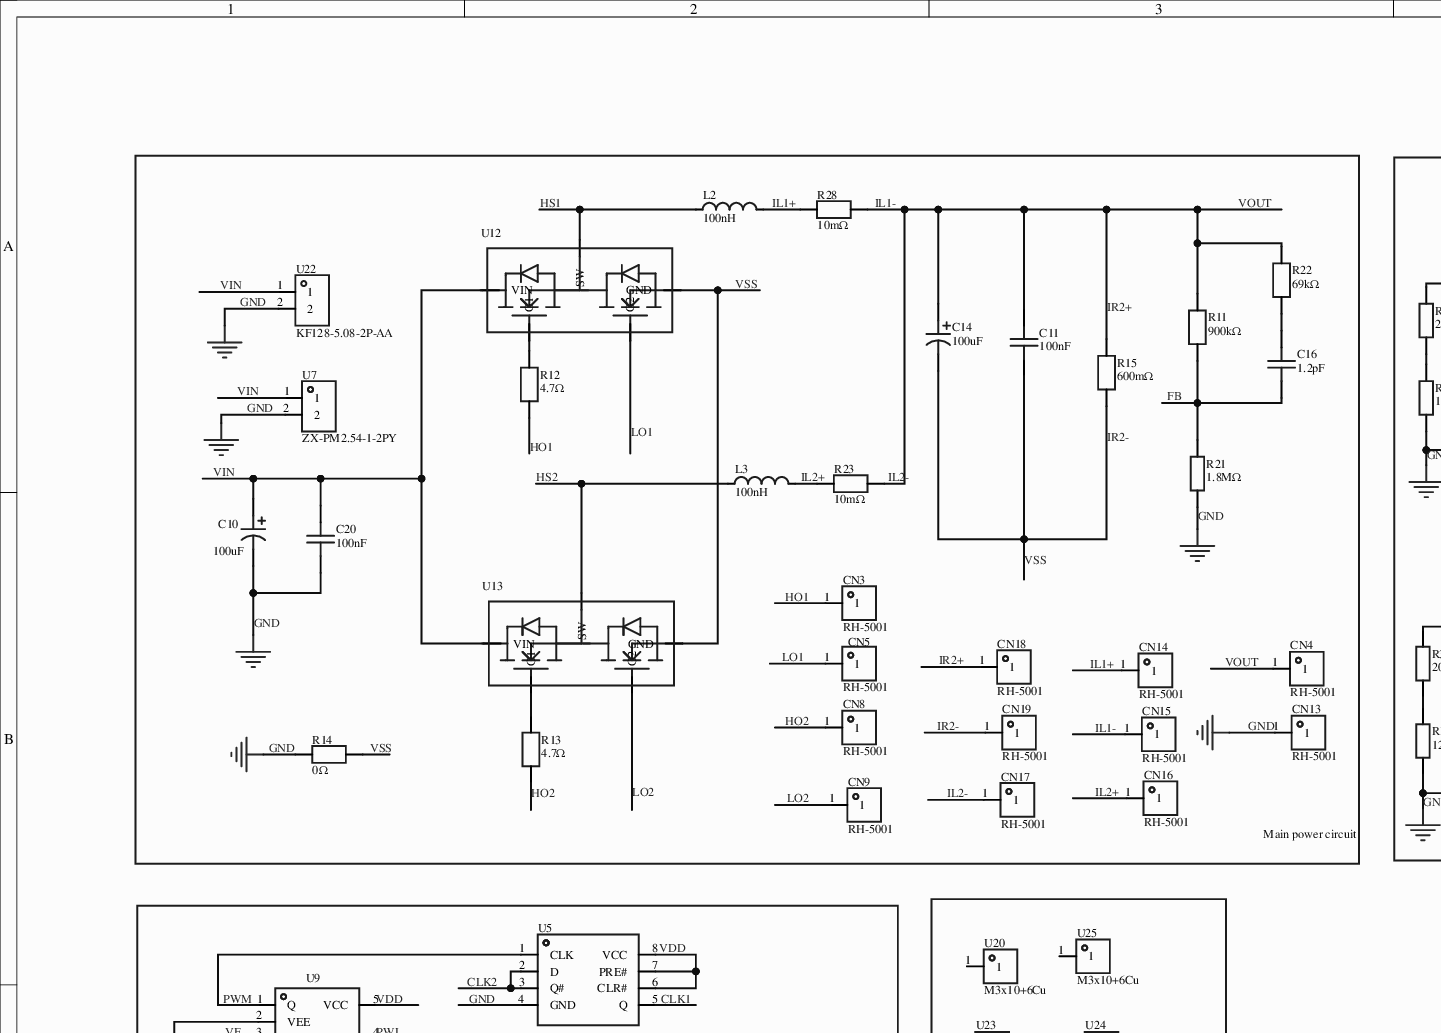
[diagram p0: MISC53275-3.schdoc, top left]
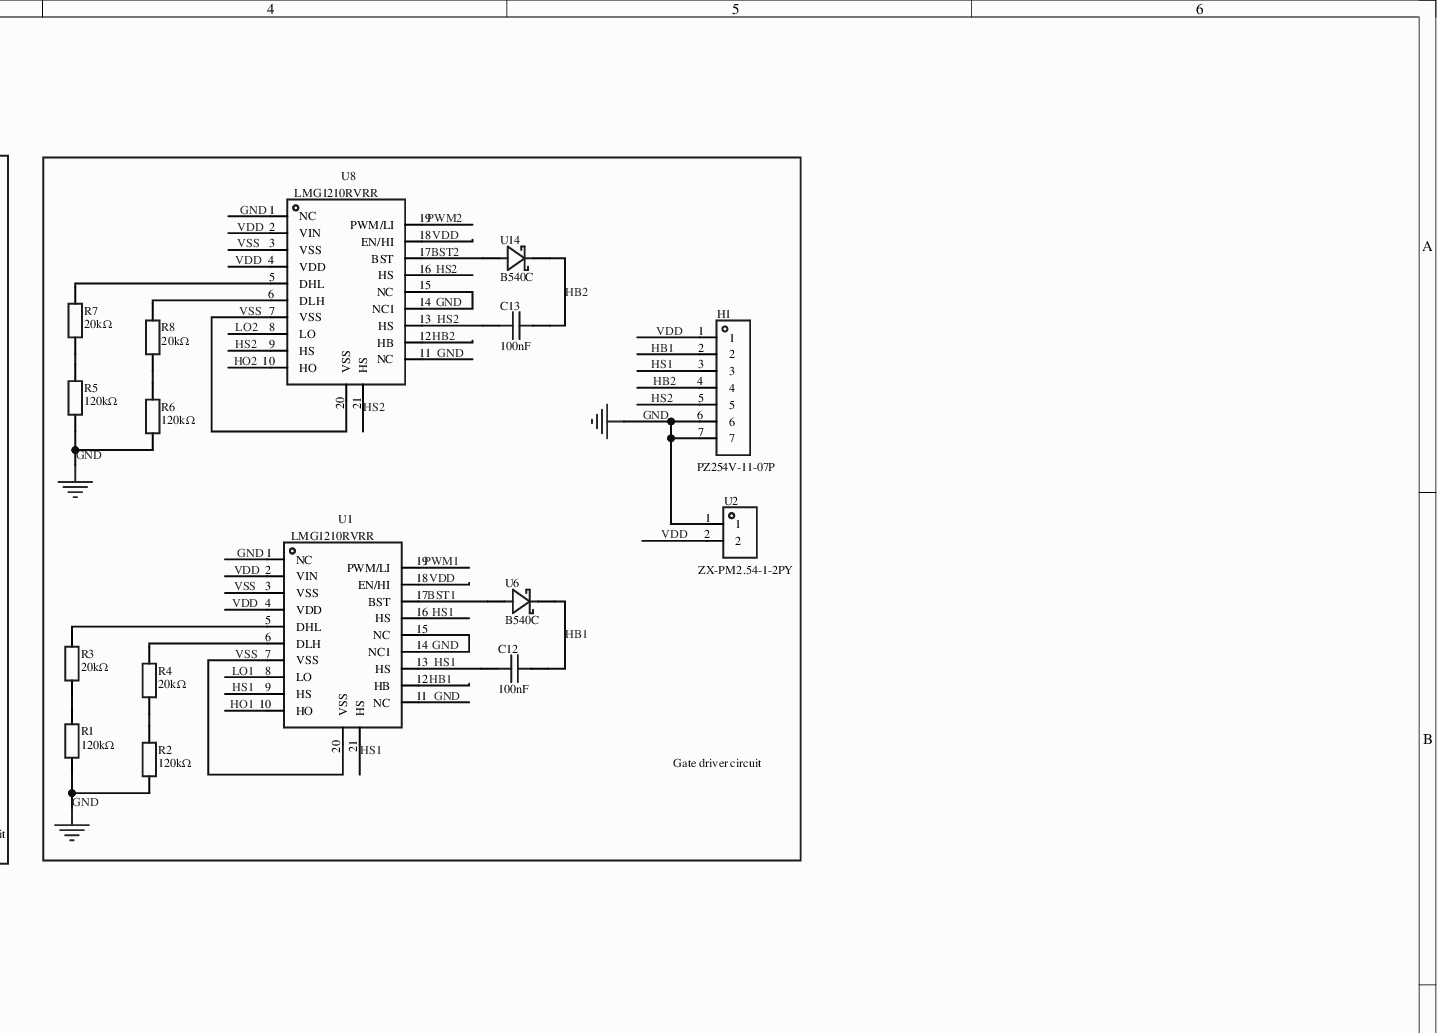
[diagram p1: MISC53275-3.schdoc, top right]
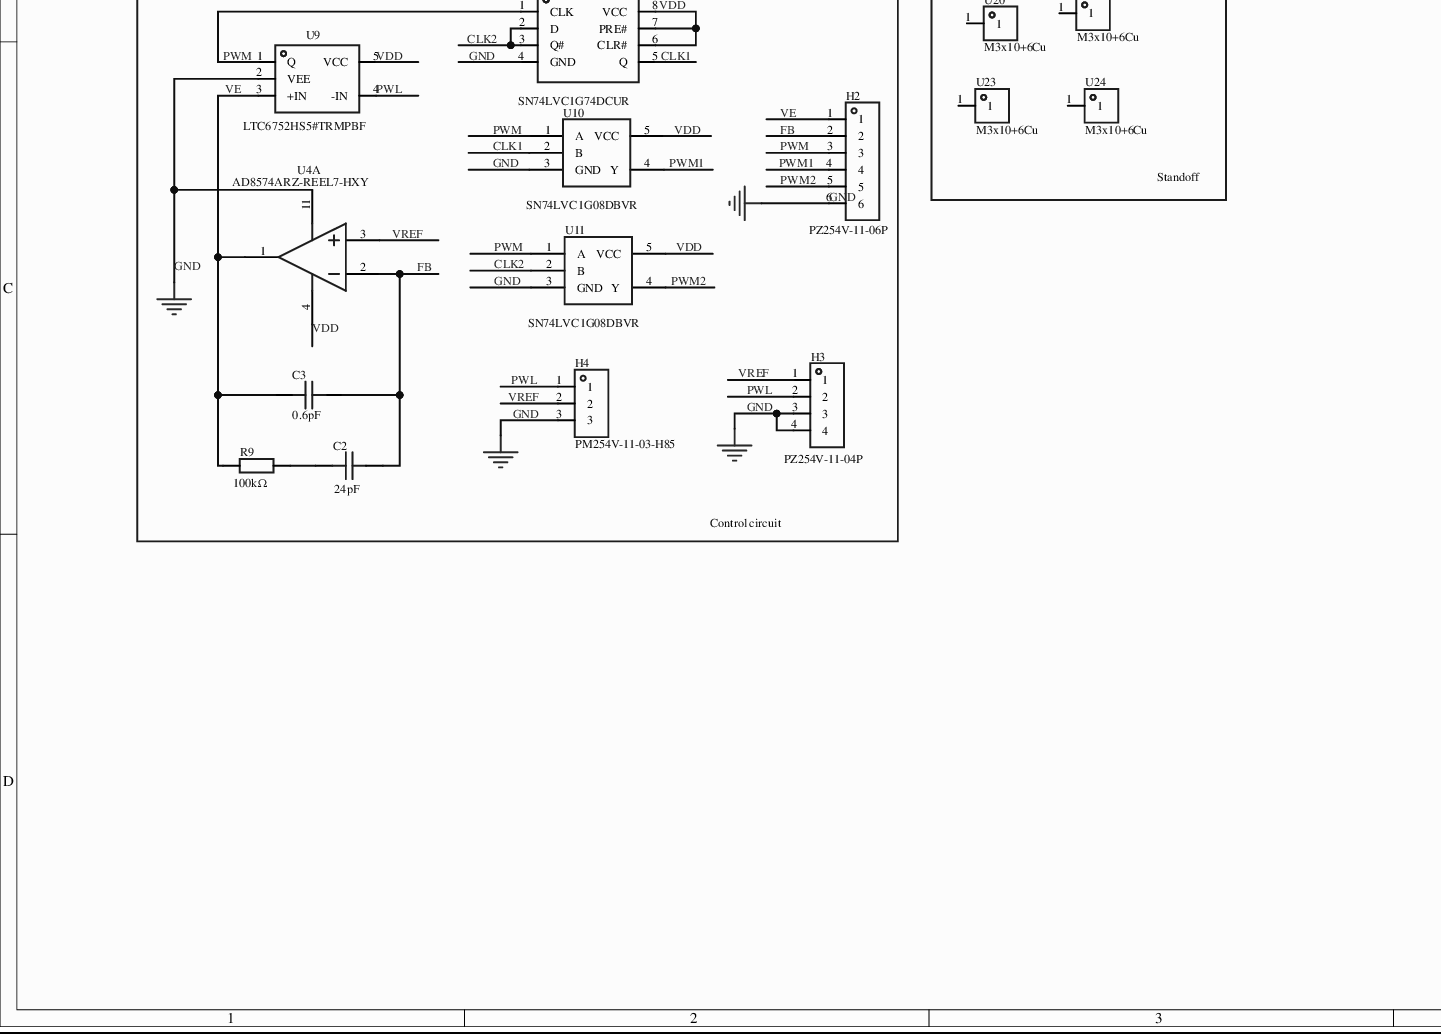
[diagram p2: MISC53275-3.schdoc, bottom left]
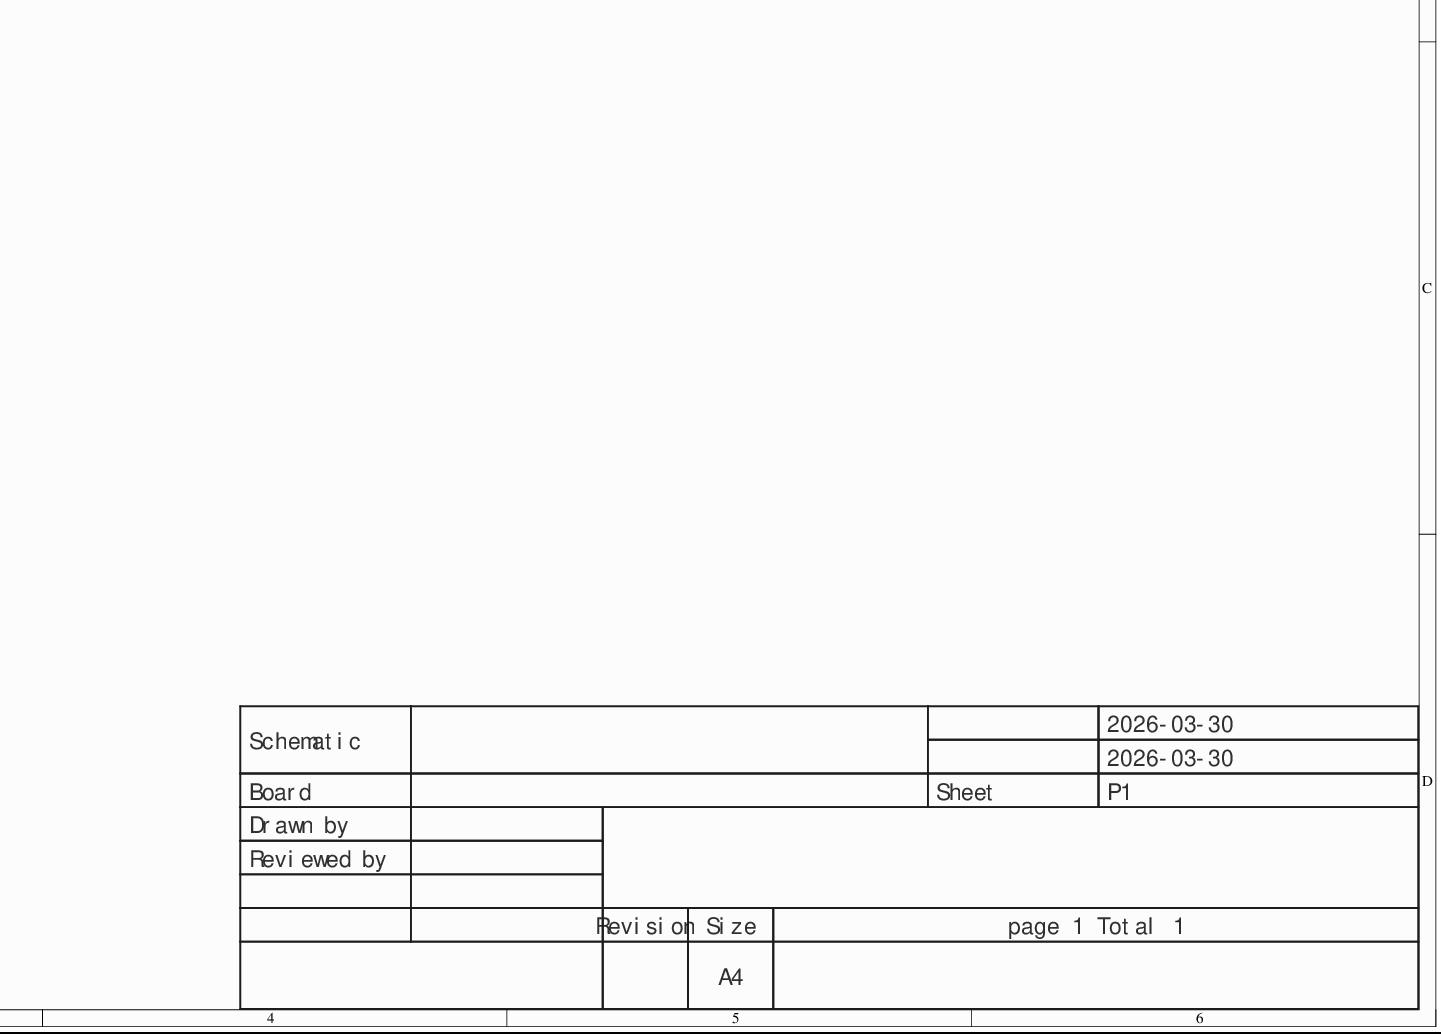
[diagram p3: MISC53275-3.schdoc, bottom right]
# Altium project MISC53275-2.PrjPcb
1 sheet, 63 parts. Net scope: global (net labels, ports and power ports of the same name join across sheets).
Board file: MISC53275.pcbdoc

## Sheet MISC53275-3.schdoc
size 420 x 297 mm; Version: V1.0; @Project Name: MISC53275; @Update Date: 2026-03-30; @Create Date: 2026-03-30; @Board Name: MISC53275; @Create Time: 11:56:40; @Page Count: 1; @Page No: 1; @Schematic Name: MISC53275; @Update Time: 11:56:40; Size: A4

### Parts
C2  24pF  [C0805]
C3  0.6pF  [C0603]
C10  100uF  [CAP-SMD_BD6.3-L6.6-W6.6-LS7.3-FD-H7.7]
C11  100nF  [CAP-SMD_L2.0-W1.25]
C12  100nF  [CAP-SMD_L2.0-W1.25]
C13  100nF  [CAP-SMD_L2.0-W1.25]
C14  100uF  [CAP-SMD_BD6.3-L6.6-W6.6-RD]
C16  1.2pF  [C0805]
C20  100nF  [CAP-SMD_L2.0-W1.25]
CN3  RH-5001  [TEST-TH_BD2.54-P1.4_BLACK]
CN4  RH-5001  [TEST-TH_BD2.54-P1.4_BLACK]
CN5  RH-5001  [TEST-TH_BD2.54-P1.4_BLACK]
CN8  RH-5001  [TEST-TH_BD2.54-P1.4_BLACK]
CN9  RH-5001  [TEST-TH_BD2.54-P1.4_BLACK]
CN13  RH-5001  [TEST-TH_BD2.54-P1.4_BLACK]
CN14  RH-5001  [TEST-TH_BD2.54-P1.4_BLACK]
CN15  RH-5001  [TEST-TH_BD2.54-P1.4_BLACK]
CN16  RH-5001  [TEST-TH_BD2.54-P1.4_BLACK]
CN17  RH-5001  [TEST-TH_BD2.54-P1.4_BLACK]
CN18  RH-5001  [TEST-TH_BD2.54-P1.4_BLACK]
CN19  RH-5001  [TEST-TH_BD2.54-P1.4_BLACK]
H1  PZ254V-11-07P  [HDR-TH_7P-P2.54-V-M]
H2  PZ254V-11-06P  [HDR-TH_6P-P2.54-V-M]
H3  PZ254V-11-04P  [HDR-TH_4P-P2.54-V-M]
H4  PM254V-11-03-H85  [HDR-TH_3P-P2.54-V-F]
L2  100nH  [IND-SMD_L2.3-W1.8]
L3  100nH  [IND-SMD_L2.3-W1.8]
R1  120kΩ  [R0805]
R2  120kΩ  [R0805]
R3  20kΩ  [R0805]
R4  20kΩ  [R0805]
R5  120kΩ  [R0805]
R6  120kΩ  [R0805]
R7  20kΩ  [R0805]
R8  20kΩ  [R0805]
R9  100kΩ  [R0805]
R11  900kΩ  [R1206]
R12  4.7Ω  [R0805]
R13  4.7Ω  [R0805]
R14  0Ω  [R1206]
R15  600mΩ  [R1206]
R21  1.8MΩ  [R0805]
R22  69kΩ  [R0603]
R23  10mΩ  [R0805]
R28  10mΩ  [R0805]
U1  LMG1210RVRR  [WQFN-19_L4.0-W3.0-P0.50-BL-EP_LMG1210RVRR]
U2  ZX-PM2.54-1-2PY  [HDR-TH_2P-P2.54-V-F]
U4  AD8574ARZ-REEL7-HXY  [SOP-14_L8.7-W3.9-P1.27-LS6.0-BL]  (part A of 4)
U5  SN74LVC1G74DCUR  [SSOP-8_L2.0-W2.3-P0.50-LS3.1-BR]
U6  B540C  [SMC_L6.9-W5.9-LS7.9-RD]
U7  ZX-PM2.54-1-2PY  [HDR-TH_2P-P2.54-V-F]
U8  LMG1210RVRR  [WQFN-19_L4.0-W3.0-P0.50-BL-EP_LMG1210RVRR]
U9  LTC6752HS5#TRMPBF  [SOT-23-5_L3.0-W1.7-P0.95-LS2.8-BL]
U10  SN74LVC1G08DBVR  [SOT-23-5_L3.0-W1.7-P0.95-LS2.8-BR]
U11  SN74LVC1G08DBVR  [SOT-23-5_L3.0-W1.7-P0.95-LS2.8-BR]
U12  (no value)  [2111]
U13  (no value)  [2111]
U14  B540C  [SMC_L6.9-W5.9-LS7.9-RD]
U20  M3x10+6Cu  [SMD_L4.7-W4.7-D3.0]
U22  KF128-5.08-2P-AA  [CONN-TH_P5.08_KF128-5.08-2P]
U23  M3x10+6Cu  [SMD_L4.7-W4.7-D3.0]
U24  M3x10+6Cu  [SMD_L4.7-W4.7-D3.0]
U25  M3x10+6Cu  [SMD_L4.7-W4.7-D3.0]

### Blocks framed on the sheet
Main power circuit: C10 C11 C14 C16 C20 CN3-CN5 CN8 CN9 CN13-CN19 L2 L3 R11-R15 R21-R23 R28 U7 U12 U13 U22
Gate driver circuit: C12 C13 H1 R1-R8 U1 U2 U6 U8 U14
Control circuit: C2 C3 H2-H4 R9 U4 U5 U9-U11
Standoff: U20 U23-U25

### Nets
GND: C10.2 C20.1 CN13.1 H1.6 H1.7 H2.6 H3.3 H3.4 H4.3 R1.1 R2.1 R5.1 R6.1 R14.1 R21.1 U1.1(NC) U1.11(NC) U1.14(NC1) U1.15(NC) U2.1 U4.11(–VS) U5.4(GND) U7.2 U8.1(NC) U8.11(NC) U8.14(NC1) U8.15(NC) U9.2(VEE) U10.3(GND) U11.3(GND) U22.2
BST1: U1.17(BST) U6.2(A)
BST2: U8.17(BST) U14.2(A)
CLK1: U5.5(Q) U10.2(B)
CLK2: U5.2(D) U5.3(Q#) U11.2(B)
FB: C2.2 C3.2 C16.1 H2.2 R11.1 R21.2 U4.2(-INA)
HB1: C12.2 H1.2 U1.12(HB) U6.1(C)
HB2: C13.2 H1.4 U8.12(HB) U14.1(C)
HO1: CN3.1 R12.1 U1.10(HO)
HO2: CN8.1 R13.1 U8.10(HO)
HS1: C12.1 H1.3 L2.1 U1.9(HS) U1.13(HS) U1.16(HS) U1.21(HS) U12.5(SW)
HS2: C13.1 H1.5 L3.1 U8.9(HS) U8.13(HS) U8.16(HS) U8.21(HS) U13.5(SW)
IL1+: CN14.1 L2.2 R28.1
IL1-: C11.2 C14.1 CN4.1 CN15.1 CN17.1 CN18.1 R11.2 R15.2 R22.2 R23.2 R28.2  [also labelled IL2-, IR2+, VOUT]
IL2+: CN16.1 L3.2 R23.1
IR2-: C11.1 C14.2 CN19.1 R14.2 R15.1 U1.3(VSS) U1.7(VSS) U1.20(VSS) U8.3(VSS) U8.7(VSS) U8.20(VSS) U12.4(GND) U13.4(GND)  [also labelled VSS]
LO1: CN5.1 U1.8(LO) U12.3(G2)
LO2: CN9.1 U8.8(LO) U13.3(G2)
PWL: H3.2 H4.1 U9.4(-IN)
PWM: H2.3 U5.1(CLK) U9.1(Q) U10.1(A) U11.1(A)
PWM1: H2.4 U1.19(PWM/LI) U10.4(Y)
PWM2: H2.5 U8.19(PWM/LI) U11.4(Y)
VDD: H1.1 U1.2(VIN) U1.4(VDD) U1.18(EN/HI) U2.2 U4.4(+VS) U5.6(CLR#) U5.7(PRE#) U5.8(VCC) U8.2(VIN) U8.4(VDD) U8.18(EN/HI) U9.5(VCC) U10.5(VCC) U11.5(VCC)
VE: C3.1 H2.1 R9.1 U4.1(OUTA) U9.3(+IN)
VIN: C10.1 C20.2 U7.1 U12.2(VIN) U13.2(VIN) U22.1
VREF: H3.1 H4.2 U4.3(+INA)
NetC2_1: C2.1 R9.2
NetC16_2: C16.2 R22.1
NetR1_2: R1.2 R3.1
NetR2_2: R2.2 R4.1
NetR3_2: R3.2 U1.5(DHL)
NetR4_2: R4.2 U1.6(DLH)
NetR5_2: R5.2 R7.1
NetR6_2: R6.2 R8.1
NetR7_2: R7.2 U8.5(DHL)
NetR8_2: R8.2 U8.6(DLH)
NetR12_2: R12.2 U12.1(G1)
NetR13_2: R13.2 U13.1(G1)

Not connected (* = marked no-connect by the designer): U20 1*; U23 1*; U24 1*; U25 1*

### Notes on the sheet
- 2026-03-30
- Schematic
- Board
- Sheet
- P1
- Drawn by
- Reviewed by
- Revision
- Size
- A4
- page 1 Total 1

### Library data of the parts
C2 = CC0805FRNPO9BN240: Capacitance: 24pF; tolerance: ±1%; rated voltage: 50V; temperature coefficient: NP0;; Manufacturer: YAGEO(国巨); 3D Model: 1ba041120af144c991958decab20d241; 3D Model Transform: 78.74,51.181,0,0,0,0,0,0.0005,0; AddInBom: yes; ModelName: C0805_L2.0-W1.3-H1.3; Symbol: CC0805FRNPO9BN240; Device: CC0805FRNPO9BN240; LCSC Part Name: 24pF ±1% 50V; Supplier Part: C527082; Manufacturer Part: CC0805FRNPO9BN240; Supplier Footprint: 0805; JLCPCB Part Class: Extended library; Datasheet: https://example.com/datasheet/CC0805FRNPO9BN240/545508.html; Supplier: LCSC; Value: 24pF; Tolerance: ±1%; Voltage Rating: 50V; Temperature Coefficient: NP0; ConvertToPcb: yes; FootprintName: C0805
C3 = GRM1885C1HR60WA01D: Capacitance: 0.6pF; rated voltage: 50V; temperature coefficient: C0G;; Manufacturer: muRata(村田); 3D Model: ac125912035d415993ca9572d50418b10819f05c4eef4c71ace90d822a990e87; 3D Model Transform: 62.992,31.496,0,0,0,0,0,0,0; AddInBom: yes; ModelName: C0603_L1.6-W0.8-H0.8; Symbol: GRM1885C1HR60WA01D; Device: GRM1885C1HR60WA01D; LCSC Part Name: ±0.05pF 0.6pF 50V; Supplier Part: C415380; Manufacturer Part: GRM1885C1HR60WA01D; Supplier Footprint: 0603; JLCPCB Part Class: Extended Part; Datasheet: https://example.com/datasheet/GRM1885C1HR60WA01D/407975.html; Supplier: LCSC; Value: 0.6pF; Voltage Rating: 50V; Temperature Coefficient: C0G; ConvertToPcb: yes; FootprintName: C0603
C10 = JVJ50V100M6x8: Capacitance: 100uF; tolerance: ±20%; rated voltage: 50V; ripple current: 140mA@120Hz;; Manufacturer: JIERR(捷而瑞); 3D Model: ccbda52dceed4b139172c40f75c9da3f0819f05c4eef4c71ace90d822a990e87; 3D Model Transform: 287.401,259.842,0,0,0,0,0,0,0; Lifetime: 2000hrs@105℃; AddInBom: yes; Symbol: JVJ50V100M6X8; Device: JVJ50V100M6x8; LCSC Part Name: 100uF ±20% 50V; Supplier Part: C46550415; Manufacturer Part: JVJ50V100M6x8; Supplier Footprint: SMD,D6.3xL7.7mm; JLCPCB Part Class: Extended Part; Datasheet: https://example.com/datasheet/JVJ50V100M6x8/48680109.html; Supplier: LCSC; Value: 100uF; Tolerance: ±20%; Voltage Rating: 50V; Ripple Current: 140mA@120Hz; Diameter: 6.3mm; Height - Seated (Max): 7.7mm; Operating Temperature: -55℃~+105℃; ConvertToPcb: yes; FootprintName: CAP-SMD_BD6.3-L6.6-W6.6-LS7.3-FD-H7.7; ModelName: CAP-SMD_BD6.3-L6.6-W6.6-LS7.3-FD-H7.7
C11-C13 C20 = FCC0805B104K500DT: Capacitance: 100nF; tolerance: ±10%; rated voltage: 50V; temperature coefficient: X7R;; Manufacturer: FOJAN(富捷); 3D Model: dce19e309e9b4209af79576cb8c62f2f; 3D Model Transform: 78.74,49.2125,0,0,0,0,0,0,0; AddInBom: yes; ModelName: CAP-SMD_L2.0-W1.3-H1.3; Symbol: FCC0805B104K500DT; Device: FCC0805B104K500DT; LCSC Part Name: 100nF ±10% 50V; Supplier Part: C5137467; Manufacturer Part: FCC0805B104K500DT; Supplier Footprint: 0805; JLCPCB Part Class: Extended Part; Datasheet: https://example.com/datasheet/FCC0805B104K500DT/5746969.html; Supplier: LCSC; Value: 100nF; Tolerance: ±10%; Voltage Rating: 50V; Temperature Coefficient: X7R; ConvertToPcb: yes; FootprintName: CAP-SMD_L2.0-W1.25
C14 = MA35V100M6X8: Capacitance: 100uF; tolerance: ±20%; rated voltage: 35V; ripple current: 2.9A@100kHz; equivalent series resistance (ESR): 30mΩ@100kHz; type: polymer;; Manufacturer: JIERR(捷而瑞); 3D Model: 901941a22e384f799727a46cfda771740819f05c4eef4c71ace90d822a990e87; 3D Model Transform: 307.086,259.842,0,0,0,0,0,0,0; Lifetime: 2000hrs@105℃; AddInBom: yes; ModelName: CAP-SMD_L6.6-W6.6-H7.0-LS7.2; Symbol: MA35V100M6X8; Device: MA35V100M6X8; LCSC Part Name: 100uF ±20% 35V; Supplier Part: C46550467; Manufacturer Part: MA35V100M6X8; Supplier Footprint: SMD,D6.3xL7.7mm; JLCPCB Part Class: Extended Part; Datasheet: https://example.com/datasheet/MA35V100M6X8/48680161.html; Supplier: LCSC; Value: 100uF; Tolerance: ±20%; Voltage Rating: 35V; Ripple Current: 2.9A@100kHz; Equivalent Series Resistance(ESR): 30mΩ@100kHz; Type: Polymer; Diameter: 6.3mm; Height - Seated (Max): 7mm; Operating Temperature: -55℃~+105℃; ConvertToPcb: yes; FootprintName: CAP-SMD_BD6.3-L6.6-W6.6-RD
C16 = MCA08HQ1R2C251T7: Capacitance: 1.2pF; rated voltage: 250V; temperature coefficient: -;; Manufacturer: MEGSINE(兆讯); 3D Model: 1ba041120af144c991958decab20d2410819f05c4eef4c71ace90d822a990e87; 3D Model Transform: 78.74,51.181,0,0,0,0,0,0.0005,0; AddInBom: yes; ModelName: C0805_L2.0-W1.3-H1.3; Symbol: MCA08HQ1R2C251T7; Device: MCA08HQ1R2C251T7; LCSC Part Name: ±0.25pF 1.2pF 250V; Supplier Part: C42432085; Manufacturer Part: MCA08HQ1R2C251T7; Supplier Footprint: 0805; Datasheet: https://example.com/datasheet/MCA08HQ1R2C251T7/44459354.html; Supplier: LCSC; Value: 1.2pF; Voltage Rating: 250V; Temperature Coefficient: -; ConvertToPcb: yes; FootprintName: C0805
CN3-CN5 CN8 CN9 CN13-CN19 = RH-5001: Test pin, high-temperature nylon / phosphor bronze silver-plated, 5001 test point, 100x80mm; Manufacturer: 荣和; 3D Model: 3b56df8954204a2c9a7df7bc4a4fe0820819f05c4eef4c71ace90d822a990e87; 3D Model Transform: 98.425,98.79098,0,0,0,0,0,0,-137.795; Connector Type: Pin, through-board; Plastic Color: Black; Board Space (Diameter φ/ Length x Width): 2.5mm; AddInBom: yes; Symbol: RH-5001; Device: RH-5001; LCSC Part Name: PCB电路板测试点/测试针; Supplier Part: C5199801; Manufacturer Part: RH-5001; Supplier Footprint: -; JLCPCB Part Class: Extended Part; Datasheet: https://example.com/upload/public/pdf/source/20240125/4C7D900D13ECC10386B63F24462DBAAB.pdf; Supplier: LCSC; ConvertToPcb: yes; FootprintName: TEST-TH_BD2.54-P1.4_BLACK; ModelName: TEST-TH_BD2.54-P1.4_BLACK
H1 = PZ254V-11-07P: Pin structure: 1x7P; pitch: 2.54mm; row spacing: -; round/square pin: square pin; mounting: through-hole; rows: single row; total pins: 7P; rated current: 3A; rated voltage: 250V; mating pin length: 6mm; plastic height: 2.5mm; termination pin length: 3mm; contact material: brass; contact plating: -; working temperature: -40℃~+105℃; color: black;; Manufacturer: XFCN(兴飞); 3D Model: 3f496cdc752348c6a5e9157bbaceaf960819f05c4eef4c71ace90d822a990e87; 3D Model Transform: 690.1561,98.425,0,0,0,0,0,0,-118.11; Circluar Pins/Square Pins: Square pins; AddInBom: yes; ModelName: HDR-TH_7P-P2.54-M-LI-1X7P; Symbol: PZ254V-11-07P; Device: PZ254V-11-07P; LCSC Part Name: 1x7P 间距:2.54mm 方针 直插; Supplier Part: C492406; Manufacturer Part: PZ254V-11-07P; Supplier Footprint: 插件,P=2.54mm; JLCPCB Part Class: Extended Part; Datasheet: https://example.com/datasheet/PZ254V-11-07P/502962.html; Supplier: LCSC; Pin Structure: 1x7P; Pitch: 2.54mm; Row Spacing: -; Mounting Type: Through-hole; Number of Rows: Single row; Number of Pins: 7P; Current Rating: 3A; Voltage Rating (Max): 250V; Length of Mating Pin: 6mm; Insulation Height: 2.5mm; Length of End Connection Pin: 3mm; Contact Material: Brass; Contact Plating: -; Operating Temperature: -40℃~+105℃; Color: Black; ConvertToPcb: yes; FootprintName: HDR-TH_7P-P2.54-V-M
H2 = PZ254V-11-06P: Pin structure: 1x6P; pitch: 2.54mm; row spacing: -; round/square pin: square pin; mounting: through-hole; rows: single row; total pins: 6P; rated current: 3A; rated voltage: 250V; mating pin length: 6mm; plastic height: 2.5mm; termination pin length: 3mm; contact material: brass; contact plating: -; working temperature: -40℃~+105℃; color: black;; Manufacturer: XFCN(兴飞); 3D Model: 66a147c6933d4029b68665bbcd1e29240819f05c4eef4c71ace90d822a990e87; 3D Model Transform: 590.1563,98.425,0,0,0,0,0,0,-118.11; Circluar Pins/Square Pins: Square pins; AddInBom: yes; ModelName: HDR-TH_6P-P2.54-M-LI-1X6P; Symbol: PZ254V-11-06P; Device: PZ254V-11-06P; LCSC Part Name: 1x6P 间距:2.54mm 方针 直插; Supplier Part: C492405; Manufacturer Part: PZ254V-11-06P; Supplier Footprint: 插件,P=2.54mm; JLCPCB Part Class: Extended Part; Datasheet: https://example.com/datasheet/PZ254V-11-06P/502961.html; Supplier: LCSC; Pin Structure: 1x6P; Pitch: 2.54mm; Row Spacing: -; Mounting Type: Through-hole; Number of Rows: Single row; Number of Pins: 6P; Current Rating: 3A; Voltage Rating (Max): 250V; Length of Mating Pin: 6mm; Insulation Height: 2.5mm; Length of End Connection Pin: 3mm; Contact Material: Brass; Contact Plating: -; Operating Temperature: -40℃~+105℃; Color: Black; ConvertToPcb: yes; FootprintName: HDR-TH_6P-P2.54-V-M
H3 = PZ254V-11-04P: Pin structure: 1x4P; pitch: 2.54mm; row spacing: -; round/square pin: square pin; mounting: through-hole; rows: single row; total pins: 4P; rated current: 3A; rated voltage: 250V; mating pin length: 6mm; plastic height: 2.5mm; termination pin length: 3mm; contact material: -; working temperature: -40℃~+105℃; color: black;; Manufacturer: XFCN(兴飞); Symbol: PZ254V-11-04P_C2691448; 3D Model: 112f4d05e8d64e99ab9a333894bea4f90819f05c4eef4c71ace90d822a990e87; 3D Model Transform: 399.999,104.7242,0,0,0,0,0,0,-118.11; Circluar Pins/Square Pins: Square pins; AddInBom: yes; ModelName: HDR-TH_4P-P2.54-M-LI-1X4P; Device: PZ254V-11-04P; LCSC Part Name: 1x4P 间距:2.54mm 方针 直插; Supplier Part: C2691448; Manufacturer Part: PZ254V-11-04P; Supplier Footprint: 插件,P=2.54mm; JLCPCB Part Class: Extended Part; Datasheet: https://example.com/datasheet/PZ254V-11-04P/2801085.html; Supplier: LCSC; Pin Structure: 1x4P; Pitch: 2.54mm; Row Spacing: -; Mounting Type: Through-hole; Number of Rows: Single row; Number of Pins: 4P; Current Rating: 3A; Voltage Rating (Max): 250V; Length of Mating Pin: 6mm; Insulation Height: 2.5mm; Length of End Connection Pin: 3mm; Contact Material: -; Operating Temperature: -40℃~+105℃; Color: Black; ConvertToPcb: yes; FootprintName: HDR-TH_4P-P2.54-V-M
H4 = PM254V-11-03-H85: Socket structure: 1x3P; pitch: 2.54mm; row spacing: -; round/square hole: square hole; mounting: through-hole; rows: single row; total hole positions: 3P; rated current: 3A; socket direction: top; plastic height: 8.5mm; contact material: brass; contact plating: -; working temperature: -40℃~+105℃;; Manufacturer: XFCN(兴飞); 3D Model: f3b3cc5aae9641bf9e56fc160cef875b0819f05c4eef4c71ace90d822a990e87; 3D Model Transform: 299.9994,100,0,0,0,0,0,0,-118.11; AddInBom: yes; ModelName: HDR2.54-F-LI-1X3P; Symbol: PM254V-11-03-H85; Device: PM254V-11-03-H85; LCSC Part Name: 1x3P 间距:2.54mm 直插; Supplier Part: C541850; Manufacturer Part: PM254V-11-03-H85; Supplier Footprint: 插件,P=2.54mm; JLCPCB Part Class: Extended Part; Datasheet: https://example.com/datasheet/PM254V-11-03-H85/562471.html; Supplier: LCSC; Holes Structure: 1x3P; Pitch: 2.54mm; Row Spacing: -; Circular Hole / Square Hole: Square hole; Mounting Type: Through-hole; Number of Rows: Single row; Number of Positions: 3P; Current Rating: 3A; Holes Direction: Top; Insulation Height: 8.5mm; Contact Material: Brass; Contact Plating: -; Operating Temperature: -40℃~+105℃; ConvertToPcb: yes; FootprintName: HDR-TH_3P-P2.54-V-F
L2 L3 = AHW2012C-R10JTF: Inductance: 100nH; tolerance: ±5%; rated current: 400mA; DC resistance (DCR): 460mΩ;; Manufacturer: APV(爱普微); 3D Model: fbcac761ab1a4de4871c2fb54fd4664a0819f05c4eef4c71ace90d822a990e87; 3D Model Transform: 90.551,66.929,0,0,0,0,0,0,0; Q @ Frequency: 65@500MHz; Frequency - Self Resonant: 1.25GHz; Type: Wirewound chip inductor; AddInBom: yes; ModelName: IND-SMD_L2.3-W1.7-H1.6; Symbol: AHW2012C-R10JTF; Device: AHW2012C-R10JTF; LCSC Part Name: 100nH ±5% 公制尺寸:2012; Supplier Part: C6808047; Manufacturer Part: AHW2012C-R10JTF; Supplier Footprint: 0805; JLCPCB Part Class: Extended Part; Datasheet: https://example.com/datasheet/AHW2012C-R10JTF/7769627.html; Supplier: LCSC; Value: 100nH; Tolerance: ±5%; Current Rating: 400mA; DC Resistance(DCR): 460mΩ; ConvertToPcb: yes; FootprintName: IND-SMD_L2.3-W1.8
R1 R2 R5 R6 = 0805W8F1203T5E: Resistor type: thick film resistor; resistance: 120kΩ; tolerance: ±1%; power: 125mW; working voltage: 150V; temperature coefficient: ±100ppm/℃;; Manufacturer: UNI-ROYAL(厚声); 3D Model: 37a81e68749a4138bd2dfa6897b24b85; 3D Model Transform: 78.74,51.181,0,0,0,0,0,-0.0005,0; AddInBom: yes; ModelName: R0805_L2.0-W1.3-H0.6; Symbol: 0805W8F1203T5E; Device: 0805W8F1203T5E; LCSC Part Name: 120kΩ ±1% 125mW 厚膜电阻; Supplier Part: C17436; Manufacturer Part: 0805W8F1203T5E; Supplier Footprint: 0805; JLCPCB Part Class: Extended library; Datasheet: https://example.com/datasheet/0805W8F1203T5E/18124.html; Supplier: LCSC; Type: Thick film resistor; Value: 120kΩ; Tolerance: ±1%; Power(Watts): 125mW; Voltage-Supply(Max): 150V; Temperature Coefficient: ±100ppm/℃; Operating Temperature: -55℃~+155℃; ConvertToPcb: yes; FootprintName: R0805
R3 R4 R7 R8 = 0805W8F2002T5E: Resistor type: thick film resistor; resistance: 20kΩ; tolerance: ±1%; power: 125mW; maximum working voltage: 150V; temperature coefficient: ±100ppm/℃;; Manufacturer: UNI-ROYAL(厚声); 3D Model: 37a81e68749a4138bd2dfa6897b24b85; 3D Model Transform: 78.74,51.181,0,0,0,0,0,-0.0005,0; AddInBom: yes; ModelName: R0805_L2.0-W1.3-H0.6; Symbol: 0805W8F2002T5E; Device: 0805W8F2002T5E; LCSC Part Name: 20kΩ ±1% 125mW 厚膜电阻; Supplier Part: C4328; Manufacturer Part: 0805W8F2002T5E; Supplier Footprint: 0805; JLCPCB Part Class: Basic library; Datasheet: https://example.com/upload/public/pdf/source/20200306/C422600_1E6D84923E4A46A82E41ADD87F860B5C.pdf; Supplier: LCSC; Type: Thick film resistor; Value: 20kΩ; Tolerance: ±1%; Power(Watts): 125mW; Overload Voltage (Max): 150V; Temperature Coefficient: ±100ppm/℃; Operating Temperature Range: -55℃~+155℃; ConvertToPcb: yes; FootprintName: R0805
R9 = 0805W8F1003T5E: Resistor type: thick film resistor; resistance: 100kΩ; tolerance: ±1%; power: 125mW; working voltage: 150V; temperature coefficient: ±100ppm/℃;; Manufacturer: UNI-ROYAL(厚声); Symbol: 0805W8F1003T5E_C149504; 3D Model: 37a81e68749a4138bd2dfa6897b24b85; 3D Model Transform: 78.74,51.181,0,0,0,0,0,-0.0005,0; AddInBom: yes; ModelName: R0805_L2.0-W1.3-H0.6; Device: 0805W8F1003T5E; LCSC Part Name: 100kΩ ±1% 125mW 厚膜电阻; Supplier Part: C149504; Manufacturer Part: 0805W8F1003T5E; Supplier Footprint: 0805; JLCPCB Part Class: Basic library; Datasheet: https://example.com/datasheet/0805W8F1003T5E/160838.html; Supplier: LCSC; Type: Thick film resistor; Value: 100kΩ; Tolerance: ±1%; Power(Watts): 125mW; Voltage-Supply(Max): 150V; Temperature Coefficient: ±100ppm/℃; Operating Temperature: -55℃~+155℃; ConvertToPcb: yes; FootprintName: R0805
R11 = RT1206BRE07900KL: Resistor type: thin film resistor; resistance: 900kΩ; tolerance: ±0.1%; power: 250mW; temperature coefficient: ±50ppm/℃;; Manufacturer: YAGEO(国巨); 3D Model: 89a1f13db2384da588040e0b3c55bf660819f05c4eef4c71ace90d822a990e87; 3D Model Transform: 125.984,62.992,0,0,0,0,0,0,0; AddInBom: yes; ModelName: R1206_L3.2-W1.6-H0.6; Symbol: RT1206BRE07900KL; Device: RT1206BRE07900KL; LCSC Part Name: 薄膜电阻 900kΩ ±0.1% 250mW; Supplier Part: C871499; Manufacturer Part: RT1206BRE07900KL; Supplier Footprint: 1206; JLCPCB Part Class: Extended Part; Datasheet: https://example.com/datasheet/RT1206BRE07900KL/931594.html; Supplier: LCSC; Type: Thin film resistor; Value: 900kΩ; Tolerance: ±0.1%; Power(Watts): 250mW; Temperature Coefficient: ±50ppm/℃; Operating Temperature: -55℃~+155℃; ConvertToPcb: yes; FootprintName: R1206
R12 R13 = FRC0805J4R7 TS: Resistor type: thick film resistor; resistance: 4.7Ω; tolerance: ±5%; power: 125mW; working voltage: 150V; temperature coefficient: ±200ppm/℃;; Manufacturer: FOJAN(富捷); 3D Model: 37a81e68749a4138bd2dfa6897b24b850819f05c4eef4c71ace90d822a990e87; 3D Model Transform: 78.74,51.181,0,0,0,0,0,-0.0005,0; AddInBom: yes; ModelName: R0805_L2.0-W1.3-H0.6; Symbol: FRC0805J4R7 TS; Device: FRC0805J4R7 TS; LCSC Part Name: 4.7Ω ±5% 125mW 厚膜电阻; Supplier Part: C2907327; Manufacturer Part: FRC0805J4R7 TS; Supplier Footprint: 0805; JLCPCB Part Class: Extended Part; Datasheet: https://example.com/datasheet/FRC0805J4R7%2520TS/3180840.html; Supplier: LCSC; Type: Thick film resistor; Value: 4.7Ω; Tolerance: ±5%; Power(Watts): 125mW; Voltage-Supply(Max): 150V; Temperature Coefficient: ±200ppm/℃; Operating Temperature: -55℃~+155℃; ConvertToPcb: yes; FootprintName: R0805
R14 = RE1206F1R000: Resistor type: sampling resistor; alloy resistor; resistance: 0Ω; tolerance: ±1%; power: 1W; mounting: SMD;; Manufacturer: JIERR(捷而瑞); 3D Model: 89a1f13db2384da588040e0b3c55bf660819f05c4eef4c71ace90d822a990e87; 3D Model Transform: 125.984,62.992,0,0,0,0,0,0,0; AddInBom: yes; ModelName: R1206_L3.2-W1.6-H0.6; Symbol: RE1206F1R000; Device: RE1206F1R000; LCSC Part Name: 0mΩ 1W 1206 ±1%; Supplier Part: C46961765; Manufacturer Part: RE1206F1R000; Supplier Footprint: 1206; JLCPCB Part Class: Extended Part; Datasheet: https://example.com/datasheet/RE1206F1R000/49133304.html; Supplier: LCSC; Type: Sampling resistor; alloy resistor; Value: 0Ω; Tolerance: ±1%; Power(Watts): 1W; Mounting Type: SMD; ConvertToPcb: yes; FootprintName: R1206
R15 = FRL1206FR600TS: Resistor type: thick film resistor; resistance: 600mΩ; tolerance: ±1%; power: 250mW; working voltage: 500V; temperature coefficient: ±200ppm/℃;; Manufacturer: FOJAN(富捷); 3D Model: 89a1f13db2384da588040e0b3c55bf660819f05c4eef4c71ace90d822a990e87; 3D Model Transform: 125.984,62.992,0,0,0,0,0,0,0; AddInBom: yes; ModelName: R1206_L3.2-W1.6-H0.6; Symbol: FRL1206FR600TS; Device: FRL1206FR600TS; LCSC Part Name: 600mΩ ±1% 250mW 厚膜电阻; Supplier Part: C2930340; Manufacturer Part: FRL1206FR600TS; Supplier Footprint: 1206; JLCPCB Part Class: Extended Part; Supplier: LCSC; Type: Thick film resistor; Value: 600mΩ; Tolerance: ±1%; Power(Watts): 250mW; Voltage-Supply(Max): 500V; Temperature Coefficient: ±200ppm/℃; Operating Temperature: -55℃~+155℃; ConvertToPcb: yes; FootprintName: R1206
R21 = 0805W8F1804T5E: Resistor type: thick film resistor; resistance: 1.8MΩ; tolerance: ±1%; power: 125mW; working voltage: 150V; temperature coefficient: ±100ppm/℃;; Manufacturer: UNI-ROYAL(厚声); 3D Model: 37a81e68749a4138bd2dfa6897b24b850819f05c4eef4c71ace90d822a990e87; 3D Model Transform: 78.74,51.181,0,0,0,0,0,-0.0005,0; AddInBom: yes; ModelName: R0805_L2.0-W1.3-H0.6; Symbol: 0805W8F1804T5E; Device: 0805W8F1804T5E; LCSC Part Name: 1.8MΩ ±1% 125mW 厚膜电阻; Supplier Part: C17399; Manufacturer Part: 0805W8F1804T5E; Supplier Footprint: 0805; JLCPCB Part Class: Extended Part; Datasheet: https://example.com/datasheet/0805W8F1804T5E/18087.html; Supplier: LCSC; Type: Thick film resistor; Value: 1.8MΩ; Tolerance: ±1%; Power(Watts): 125mW; Voltage-Supply(Max): 150V; Temperature Coefficient: ±100ppm/℃; Operating Temperature: -55℃~+155℃; ConvertToPcb: yes; FootprintName: R0805
R22 = RT0603BRD0769KL: Resistor type: thin film resistor; resistance: 69kΩ; tolerance: ±0.1%; power: 100mW; temperature coefficient: ±25ppm/℃;; Manufacturer: YAGEO(国巨); 3D Model: fc143cca1e79419f9cd78b61e9279f080819f05c4eef4c71ace90d822a990e87; 3D Model Transform: 31.8897,63.7794,0,90,0,0,0,0,0; AddInBom: yes; Symbol: RT0603BRD0769KL; Device: RT0603BRD0769KL; LCSC Part Name: 薄膜电阻 69kΩ ±0.1% 100mW; Supplier Part: C861527; Manufacturer Part: RT0603BRD0769KL; Supplier Footprint: 0603; JLCPCB Part Class: Extended Part; Datasheet: https://example.com/upload/public/pdf/source/20231208/4FA72C41188346433D85D99700271040.pdf; Supplier: LCSC; Type: Thin film resistor; Value: 69kΩ; Tolerance: ±0.1%; Power(Watts): 100mW; Temperature Coefficient: ±25ppm/℃; Operating Temperature Range: -55℃~+155℃; ConvertToPcb: yes; FootprintName: R0603; ModelName: R0603
R23 R28 = RE0805FBR010: Resistor type: alloy resistor; resistance: 10mΩ; tolerance: ±1%; power: 750mW; temperature coefficient: ±50ppm/℃; mounting: SMD;; Manufacturer: JIERR(捷而瑞); 3D Model: 37a81e68749a4138bd2dfa6897b24b850819f05c4eef4c71ace90d822a990e87; 3D Model Transform: 78.74,51.181,0,0,0,0,0,-0.0005,0; AddInBom: yes; ModelName: R0805_L2.0-W1.3-H0.6; Symbol: RE0805FBR010; Device: RE0805FBR010; LCSC Part Name: 10mΩ 0.75W 0805 ±1%; Supplier Part: C51934131; Manufacturer Part: RE0805FBR010; Supplier Footprint: 0805; JLCPCB Part Class: Extended Part; Datasheet: https://example.com/datasheet/RE0805FBR010/54649543.html; Supplier: LCSC; Type: Alloy resistor; Value: 10mΩ; Tolerance: ±1%; Power(Watts): 750mW; Temperature Coefficient: ±50ppm/℃; Mounting Type: SMD; ConvertToPcb: yes; FootprintName: R0805
U1 U8 = LMG1210RVRR: Driver configuration: half-bridge; load type: MOSFET; driver channels: 2; sink current (IOL): 3A; source current (IOH): 1.5A; working voltage: 6V~18V; rise time (tr): 500ps; fall time (tf): 2.3ns;; Manufacturer: TI(德州仪器); 3D Model: ecefcc7351bd47d987b3c025e1752eba; 3D Model Transform: 158.267,118.8974,0,0,0,0,0,0,0; Number of Drivers: 2; Propagation Delay tpLH: 10ns; Input Logic Level - High: 1.7V~2.45V; Input Logic Level - Low: 700mV~1.3V; Quiescent Current(Iq): 300uA; AddInBom: yes; Symbol: LMG1210RVRR; Device: LMG1210RVRR; LCSC Part Name: 具有可调节死区时间的半桥MOSFET和GaNFET驱动器; Supplier Part: C2677136; Manufacturer Part: LMG1210RVRR; Supplier Footprint: WQFN-19-EP(3x4); JLCPCB Part Class: Extended library; Supplier: LCSC; Driven Configuration: Half-bridge; Load Type: MOSFET; Current - Output Low(IOL): 3A; Current - Output High(IOH): 1.5A; Voltage - Supply: 6V~18V; Rise Time: 500ps; Fall Time: 2.3ns; Propagation Delay tpHL: 10ns; Features: Undervoltage protection (UVP); overtemperature protection (OTP); Operating Temperature: -40℃~+125℃; ConvertToPcb: yes; FootprintName: WQFN-19_L4.0-W3.0-P0.50-BL-EP_LMG1210RVRR; ModelName: WQFN-19_L4.0-W3.0-P0.50-BL-EP_LMG1210RVRR
U2 U7 = ZX-PM2.54-1-2PY: Socket structure: 1x2P; pitch: 2.54mm; row spacing: -; round/square hole: square hole; mounting: through-hole; rows: single row; total hole positions: 2P; rated current: 3A; rated voltage: -; socket direction: top; plastic height: 8.5mm; contact material: brass; contact plating: gold; working temperature: -40℃~+105℃;; Manufacturer: Megastar(兆星); 3D Model: a9450ef445564560a104363b9aacde4e0819f05c4eef4c71ace90d822a990e87; 3D Model Transform: 215.7476,98.425,0,0,0,0,0,0,-129.921; PIN Length: 3.2mm; AddInBom: yes; ModelName: HDR-TH_2P-P2.54-F-LI-1X2P; Symbol: ZX-PM2.54-1-2PY; Device: ZX-PM2.54-1-2PY; LCSC Part Name: 1x2P 间距:2.54mm 直插; Supplier Part: C7499322; Manufacturer Part: ZX-PM2.54-1-2PY; Supplier Footprint: 插件,P=2.54mm; JLCPCB Part Class: Extended Part; Datasheet: https://example.com/datasheet/ZX-PM2.54-1-2PY/8573983.html; Supplier: LCSC; Holes Structure: 1x2P; Pitch: 2.54mm; Row Spacing: -; Circular Hole / Square Hole: Square hole; Mounting Type: Through-hole; Number of Rows: Single row; Number of Positions: 2P; Current Rating: 3A; Voltage Rating (Max): -; Holes Direction: Top; Insulation Height: 8.5mm; Contact Material: Brass; Contact Plating: Gold; Operating Temperature: -40℃~+105℃; ConvertToPcb: yes; FootprintName: HDR-TH_2P-P2.54-V-F
U4 = AD8574ARZ-REEL7-HXY: Amplifier count: quad; gain-bandwidth product (GBP): 1.5MHz; input bias current (Ib): 70pA; input offset voltage (Vos): 2uV; slew rate (SR): 1.2V/us; rail-to-rail: rail-to-rail input, rail-to-rail output;; Manufacturer: HXY MOSFET(华轩阳电子); Relevance: []; 3D Model: 81979219354241bfb99806b876ac1c80; 3D Model Transform: 342.519,236.22,0,0,0,0,0,0,0; Common Mode Rejection Ratio(CMRR): 126dB; Output Current: 40mA; Input Offset Voltage Drift(Vos TC): 5nV/℃; Quiescent Current(Iq): 125uA; Single Supply: 1.8V~5.5V; Dual Supply: 1V~2.75V; -2.75V~-1V; Noise density(eN): 19nV/√Hz@1kHz; Input Offset Current(Ios): 700pA; AddInBom: yes; Symbol: AD8574ARZ-REEL7-HXY; Device: AD8574ARZ-REEL7-HXY; LCSC Part Name: 零漂移、微功耗1.5MHz、轨到轨输入输出运算放大器; Supplier Part: C49307760; Manufacturer Part: AD8574ARZ-REEL7-HXY; Supplier Footprint: SOP-14; JLCPCB Part Class: Extended library; Datasheet: https://example.com/datasheet/AD8574ARZ-REEL7-HXY/51772332.html; Supplier: LCSC; Number of Channels: Quad; Gain Bandwidth Product: 1.5MHz; Ib - Input Bias Current: 70pA; Vos - Input Offset Voltage: 2uV; Slew Rate: 1.2V/us; Rail to Rail: Rail-to-rail input, rail-to-rail output; Features: EMI filter/RF suppression; ESD protection; built-in compensation; zero drift/auto-zero; Operating Temperature: -40℃~+125℃; ConvertToPcb: yes; FootprintName: SOP-14_L8.7-W3.9-P1.27-LS6.0-BL; ModelName: SOP-14_L8.7-W3.9-P1.27-LS6.0-BL
U5 = SN74LVC1G74DCUR: Type: D-type; working voltage: 1.65V~5.5V; clock frequency (fc): 200MHz; number of elements: 1; bits per element: 1; propagation delay (tpd): 6.4ns@5V,50pF; quiescent current (Iq): 10uA;; Manufacturer: TI(德州仪器); Symbol: SN74LVC1G74DCUR_C70285; 3D Model: 0897d9a9aab64803ba8a74d2c6df32aa; 3D Model Transform: 122.047,78.74,0,0,0,0,0,0,0; Trigger Type: Rising edge; Function: Set and reset; Number of Elements: 1; Output Type: Complementary; Current - Output Low(IOL): 32mA; Input Capacitance: 5pF; AddInBom: yes; Device: SN74LVC1G74DCUR; LCSC Part Name: SN74LVC1G74DCUR; Supplier Part: C70285; Manufacturer Part: SN74LVC1G74DCUR; Supplier Footprint: VSSOP-8; JLCPCB Part Class: Extended library; Supplier: LCSC; Voltage - Supply: 1.65V~5.5V; Clock Frequency: 200MHz; Number of Bits per Element: 1; Propagation Delay: 6.4ns@5V,50pF; Series: 74LVC series; Current - Output High(IOH): 32mA; Quiescent Current: 10uA; Operating Temperature: -40℃~+125℃; ConvertToPcb: yes; FootprintName: SSOP-8_L2.0-W2.3-P0.50-LS3.1-BR; ModelName: SSOP-8_L2.0-W2.3-P0.50-LS3.1-BR
U6 U14 = B540C_C6807783: Diode configuration: single; forward voltage (Vf): 550mV@5A; DC reverse voltage (Vr): 40V; rectifier current: 5A;; Manufacturer: FUXINSEMI(富芯森美); 3D Model: 181deed3e51b4528a83dd624c23bafda; 3D Model Transform: 314.96,236.22,0,0,0,0,0,0,0; Reverse Leakage Current (Ir): 100uA@40V; Operating Junction Temperature Range: -55℃~+150℃; AddInBom: yes; Symbol: B540C; Device: B540C_C6807783; LCSC Part Name: 电压:40V 电流:5A; Supplier Part: C6807783; Manufacturer Part: B540C; Supplier Footprint: SMC(DO-214AB); JLCPCB Part Class: Extended library; Datasheet: https://example.com/datasheet/B540C/7769271.html; Supplier: LCSC; Diode Configuration: Single; Voltage - Forward(Vf@If): 550mV@5A; Voltage - DC Reverse(Vr): 40V; Current - Rectified: 5A; ConvertToPcb: yes; FootprintName: SMC_L6.9-W5.9-LS7.9-RD; ModelName: SMC_L6.9-W5.9-LS7.9-RD
U9 = LTC6752HS5#TRMPBF: Comparator count: single; input offset voltage (Vos): 1.2mV; input bias current (Ib): 1.35uA; rail-to-rail: rail-to-rail input;; Manufacturer: ADI(亚德诺); 3D Model: 0a2a1b8f50944f73965918ad6e5fe167; 3D Model Transform: 118.60433,114.173,0,90,0,0,0.0005,0.0005,0; Propagation Delay Time: 2.9ns; Input Hysteresis Voltage (Vhys): 5mV; Output Type: CMOS; Quiescent Current: 4.5mA; AddInBom: yes; ModelName: SOT-23-5_L2.9-W1.6-H1.1-LS2.8-P0.95; Symbol: LTC6752HS5#TRMPBF; Device: LTC6752HS5#TRMPBF; LCSC Part Name: 280MHz、2.9ns 比较器系列，具有轨到轨输入和CMOS输出; Supplier Part: C689467; Manufacturer Part: LTC6752HS5#TRMPBF; Supplier Footprint: TSOT-23-5; JLCPCB Part Class: Extended library; Datasheet: https://example.com/datasheet/LTC6752HS5%2523TRMPBF/720185.html; Supplier: LCSC; Number of Channels: Single; Vos - Input Offset Voltage: 1.2mV; Ib - Input Bias Current: 1.35uA; Common Mode Rejection Ratio(CMRR): -; Rail to Rail: Rail-to-rail input; Operating Temperature: -40℃~+125℃; ConvertToPcb: yes; FootprintName: SOT-23-5_L3.0-W1.7-P0.95-LS2.8-BL
U10 U11 = SN74LVC1G08DBVR: Logic type: AND gate; channels: 1; working voltage: 1.65V~5.5V; quiescent current (Iq): 10uA; propagation delay (tpd): 4ns@5V,50pF;; Manufacturer: TI(德州仪器); 3D Model: 0a2a1b8f50944f73965918ad6e5fe167; 3D Model Transform: 114.173,109.636,0,180,0,0,0,0,0; Number of Channels: 1; Current - Output Low(IOL): 32mA; Input Logic Level - High: 2V; 1.7V; Input Logic Level - Low: 800mV; 700mV; Output Logic Level - High: 1.9V; 2.3V; 1.2V; 3.8V; Output Logic Level - Low: 550mV; 300mV; 450mV; Input Number: 2; AddInBom: yes; ModelName: SOT-23-5_L2.9-W1.6-H1.1-LS2.8-P0.95; Symbol: SN74LVC1G08DBVR; Device: SN74LVC1G08DBVR; LCSC Part Name: 单路 2 输入正与门; Supplier Part: C7666; Manufacturer Part: SN74LVC1G08DBVR; Supplier Footprint: SOT-23-5; JLCPCB Part Class: Extended library; Supplier: LCSC; Logic Type: AND gate; Voltage - Supply: 1.65V~5.5V; Quiescent Current: 10uA; Current - Output High(IOH): 32mA; Series: 74LVC series; Propagation Delay: 4ns@5V,50pF; Operating Temperature: -40℃~+125℃; ConvertToPcb: yes; FootprintName: SOT-23-5_L3.0-W1.7-P0.95-LS2.8-BR
U12 U13 = EPC2111: AddInBom: yes; Symbol: EPC2111; Device: EPC2111; ConvertToPcb: yes; FootprintName: 2111
U20 U23-U25 = M3x10+6Cu: M3x10+6; Manufacturer: Shuntian(顺天五金); Thread length: 6mm; material quality: Brass; surface treatment: natural finish; structure type: Single head; Shape Type: Hex; purpose: Isolation; hexagonal opposite edge: 4.7mm; AddInBom: yes; Symbol: M3X10+6CU; Device: M3x10+6Cu; LCSC Part Name: Shuntian(顺天五金) 单头六角隔离铜柱螺柱 M3X10+6 国标 黄铜 袋装; Supplier Part: C551322; Manufacturer Part: M3x10+6Cu; Supplier Footprint: -; JLCPCB Part Class: Extended Part; Datasheet: https://example.com/datasheet/M3x10+6Cu/575012.html; Supplier: LCSC; length: 10mm; diameter: 3mm; pitch: -; standard: GB standard; Specifications: M3X10+6; Installation process: -; type: Stud; Length from PC board: -; strength grade: -; colour: -; ConvertToPcb: yes; FootprintName: SMD_L4.7-W4.7-D3.0
U22 = KF128-5.08-2P-AA: Structure: 1x2P; pitch: 5.08mm; color: green; mounting: through-hole; rows: 1; pins per row: 2; rated current: 24A; rated voltage: 250V; wire gauge - AWG: 12~22; wire gauge - mm²: 2.5; working temperature: -40℃~+105℃;; Manufacturer: KEFA(科发); 3D Model: be36e72b75ac4dee8d6e181eb7e8d7840819f05c4eef4c71ace90d822a990e87; 3D Model Transform: 423.625,421.259,0,180,0,0,11.811,1.378,-137.795; Number of PINs Per Row: 2; Wire Gauge - mm2: 2.5; AddInBom: yes; Symbol: KF128-5.08-2P; Device: KF128-5.08-2P-AA; LCSC Part Name: 5.08mm 1x2P 排数:1 每排P数:2 直插; Supplier Part: C474952; Manufacturer Part: KF128-5.08-2P-AA; Supplier Footprint: 插件,P=5.08mm; JLCPCB Part Class: Extended Part; Datasheet: https://example.com/datasheet/KF128-5.08-2P-AA/481570.html; Supplier: LCSC; Number of Positions or Pins: 1x2P; Pitch: 5.08mm; Color: Green; Mounting Type: Through-hole; Number of Pins: 2P; Number of Rows: 1; Current Rating: 24A; Voltage Rating (Max): 250V; Wire Gauge - AWG: 12~22; Operating Temperature: -40℃~+105℃; ConvertToPcb: yes; FootprintName: CONN-TH_P5.08_KF128-5.08-2P; ModelName: CONN-TH_P5.08_KF128-5.08-2P